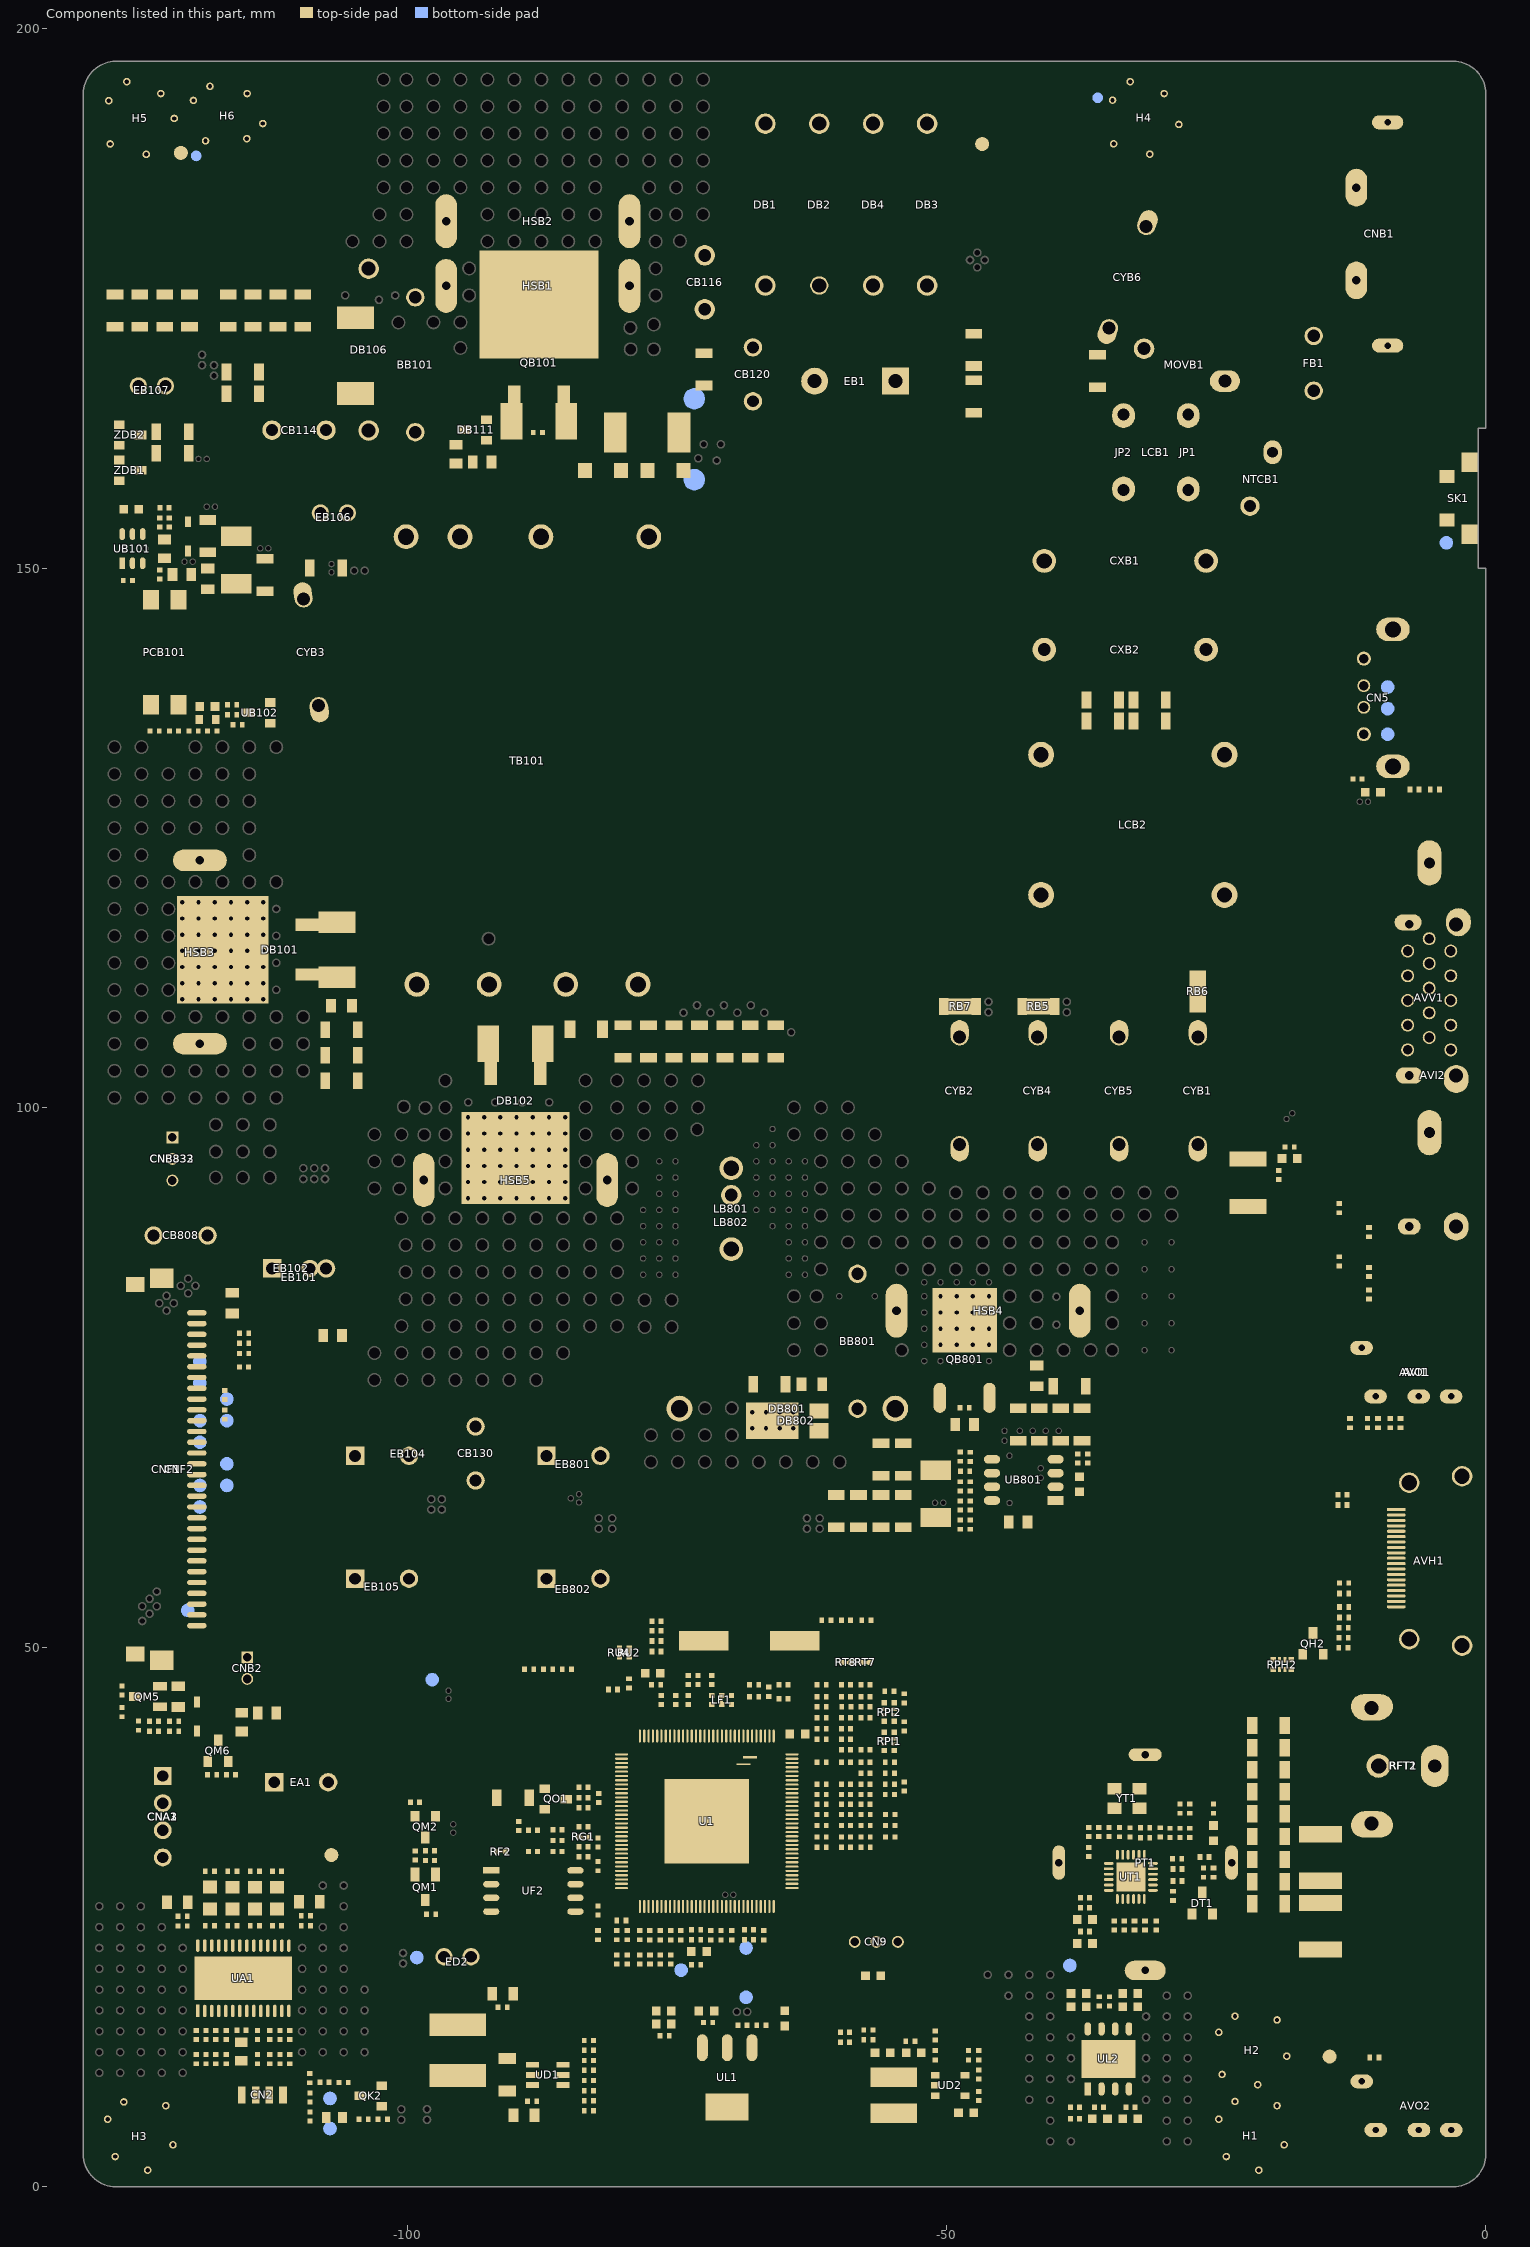
[diagram p0: the components of this part, seen from the top]
# Altium PCB MISC84438.PcbDoc (part 5 of 15)
Units mm, origin at the board's own origin, x right, y up, seen from the top; angles counter-clockwise.
Board outline 130 x 197 mm, 2 copper layers (TopLayer, BottomLayer), stack 1.571 mm thick; 574 components, 314 nets, 2636 pads, 811 vias.

## Footprints (in the part's own frame and the unit in brackets; to place one, negate y for a bottom-side part, rotate by r counter-clockwise, add the part's x,y. Pads: shape width x height; smd on the part's side, far side on the other; paste and mask are expansions set on the pad) (continued)
SIP3/2.0D-CP [mm] "捷仕泰/铭锋达;带扣插座与非带扣插座 兼容；15.07.11"
  rect 1.4x1.4 on Top Overlay: 0(-2,0)
  round 1.4 on Top Overlay: 0(0,0) 0(2,0)
  rect 1.1x1.1 hole 0.8: 1(-2,0)
  round 1.1 hole 0.8: 2(0,0) 3(2,0)
  silkscreen extent -4,-3.2 4,3.07, body extent -4,-3.2 4,1.8, height 6
SIP3H/2.0D-3 [mm] "捷仕泰：A2004AW-03-A1MA-P，带扣，加强筋"
  rect 1.6x1.6 on Top Overlay: 0(-2,0)
  round 1.6 on Top Overlay: 0(0,0) 0(2,0)
  rect 1.1x1.1 hole 0.8: 1(-2,0)
  round 1.1 hole 0.8: 2(0,0) 3(2,0)
  silkscreen extent -4.1,-7.95 4.1,1.5
SIP4/2.5D-2 [mm] "捷仕泰，A2502-04-A5WA-P（为保证与SIP4/2.54D-1兼容。改PIN间距为2.52mm，18.05.28）"
  rect 1.905x1.905 on Top Overlay: 0(-3.78,0)
  round 1.905 on Top Overlay: 0(-1.26,0) 0(1.26,0) 0(3.78,0)
  rect 1.651x1.651 hole 1.05: 1(-3.78,0)
  round 1.651 hole 1.05: 2(-1.26,0) 3(1.26,0) 4(3.78,0)
  silkscreen extent -6.4,-3.6 6.4,3
SIP4/2.54D-1 [mm] "捷仕泰/铭锋达"
  rect 1.905x1.905 on Top Overlay: 0(-3.78,0)
  round 1.905 on Top Overlay: 0(-1.26,0) 0(1.26,0) 0(3.78,0)
  rect 1.651x1.651 hole 1.05: 1(-3.78,0)
  round 1.651 hole 1.05: 2(-1.26,0) 3(1.26,0) 4(3.78,0)
  silkscreen extent -6.44,-3.5 6.44,2.5, body extent -6.35,-3.5 6.35,2.5, height 7
SIP4H/2.54D-2 [mm] "捷仕泰/铭锋达    SPEAKER"
  rect 1.905x1.905 on Top Overlay: 0(-3.78,0)
  round 1.905 on Top Overlay: 0(-1.26,0) 0(1.26,0) 0(3.78,0)
  rect 1.651x1.651 hole 1.05: 1(-3.78,0)
  round 1.651 hole 1.05: 2(-1.26,0) 3(1.26,0) 4(3.78,0)
  silkscreen extent -6.29,-7.2 6.29,0.89
SMD4532-1 [mm] "Brightking,4532-091-LF,气体放电管,雷电防护器件，17.06.12"
  rect 1.5x4 smd: 1(-2.15,0) 2(2.151,0)
  silkscreen extent -1.25,-1.79 1.23,1.71, body extent -2.41,-1.75 2.41,1.75, height 3
SO-8A [mm] "FLASH"
  rect 1.5x0.8 smd: 1(-2.95,1.905)
  oval 1.5x0.8 smd: 2(-2.95,0.635) 3(-2.95,-0.635) 4(-2.95,-1.905) 5(2.95,-1.905) 6(2.95,-0.635) 7(2.95,0.635) 8(2.95,1.905)
  silkscreen extent -4.71,-2.54 2,2.54, body extent -3.1,-2.5 3.1,2.5, height 1.76
SO-23 [mm] "双向二极管封装"
  rect 0.8x1 smd: 1(0.952,1.016) 3(-0.953,1.016)
  rect 0.8x1.1 smd: 2(0,-0.966)
  silkscreen extent -1.55,-0.86 1.55,0.36, body extent -1.5,-1.25 1.5,1.25, height 1.1
SOIC8 [mm] "W25X40BVSNIG/GD25Q32BSIG/GD25LQ16"
  rect 1.5x0.6 smd: 1(-3.9,1.905)
  oval 1.5x0.6 smd: 2(-3.9,0.635) 3(-3.9,-0.635) 4(-3.9,-1.905) 5(3.9,-1.905) 6(3.9,-0.635) 7(3.9,0.635) 8(3.9,1.905)
  silkscreen extent -5.71,-2.65 2.7,2.65, body extent -4.05,-2.69 4.05,2.69, height 2.17
SOP8/1.27-3 [mm] "LEADCHIP;LC1118;14-05-09"
  rect 1.238x0.6 smd: 1(-2.783,1.905)
  oval 1.238x0.6 smd: 2(-2.783,0.635) 3(-2.783,-0.635) 4(-2.783,-1.905) 5(2.783,-1.905) 6(2.783,-0.635) 7(2.783,0.635) 8(2.783,1.905)
  rect 3.5x5 smd paste-3 mask-3: EPAD(0,0)
  silkscreen extent -3.31,-2.5 4.16,3.42, body extent -3.1,-2.5 3.1,2.5, height 1.76
SOT-23 [mm]
  rect 0.8x1 smd: B(0.952,1.016) E(-0.953,1.016)
  rect 0.8x1.1 smd: C(-0.013,-0.966)
  silkscreen extent -1.55,-0.81 1.55,0.36, body extent -1.5,-1.25 1.5,1.25, height 1.1
SOT-23-1 [mm]
  rect 0.8x1.1 smd: D(0,-1.15)
  rect 0.8x1.27 smd: G(0.95,1.2) S(-0.95,1.2)
  TopLayer pour cut-out: -1.583,0.903 -1.583,-0.905 1.587,-0.905 1.587,0.903
  silkscreen extent -1.55,-1.05 1.55,0.33, body extent -1.52,-1.48 1.52,1.48, height 1.25
SOT-23-5 [mm] "LPW5206(1.295mm)"
  rect 0.6x0.8 smd: 1(-0.95,-1.375) 2(0,-1.375) 3(0.95,-1.375) 4(0.95,1.375) 5(-0.95,1.375)
  silkscreen extent -1.5,-2.49 1.5,0.85, body extent -1.5,-0.85 1.5,0.85, height 1.45
SOT-23-6 [mm] "RICHTEK RT9266//RT7295A(1mm)"
  rect 0.55x1.2 smd: 1(-0.95,-1.4) 2(0,-1.4) 3(0.95,-1.4) 4(0.95,1.4) 5(0,1.4) 6(-0.95,1.4)
  silkscreen extent -2.4,-1.88 1.55,0.9, body extent -1.55,-0.9 1.55,0.9, height 1.3
SOT-23-RAK [mm] "TL431G-AE2-R(UTC)"
  rect 0.8x1.1 smd: A(0.013,0.966)
  rect 0.8x1 smd: K(0.953,-1.016) R(-0.953,-1.016)
  silkscreen extent -1.52,-0.36 1.52,0.86, body extent -1.5,-1.25 1.5,1.25, height 1.1
SOT-26 [mm] "LD7536R"
  rect 0.5x1.1 smd: 1(0.95,1.35)
  oval 0.5x1.1 smd: 2(0,1.35) 3(-0.95,1.35) 4(-0.95,-1.35) 5(0,-1.35) 6(0.95,-1.35)
  silkscreen extent -1.55,-2.54 2.29,1.76, body extent -1.55,-0.9 1.55,0.9, height 1.45
SOT-223 [mm]
  oval 1x2.5 smd: 1(-2.3,-2.75) 2(0,-2.75) 3(2.3,-2.75)
  rect 4x2.5 smd: 4(0,2.75)
  TopLayer pour cut-out: 2.3,-1.188 2.3,-4.312 -2.345,-4.312 -2.64,-4.253 -2.891,-4.086 -3.058,-3.835 -3.117,-3.54 -3.117,-3.54 -2.299,-3.54 -2.299,-1.956 -3.124,-1.956 -3.066,-1.662 -2.899,-1.413 -2.65,-1.247 -2.356,-1.188 -2.356,-1.188
  silkscreen extent -3.45,-2.75 3.45,2.81, body extent -3.35,-3.3 3.35,3.4, height 1.7
SSOP28/0.65-5 [mm] "TI;TPA3140D2PWPR;15.07.08"
  rect 1.15x0.34 smd: 1(-3.025,4.225)
  oval 1.15x0.34 smd: 2(-3.025,3.575) 3(-3.025,2.925) 4(-3.025,2.275) 5(-3.025,1.625) 6(-3.025,0.975) 7(-3.025,0.325) 8(-3.025,-0.325) 9(-3.025,-0.975) 10(-3.025,-1.625) 11(-3.025,-2.275) 12(-3.025,-2.925) 13(-3.025,-3.575) 14(-3.025,-4.225) 15(3.025,-4.225) 16(3.025,-3.575) 17(3.025,-2.925) 18(3.025,-2.275) 19(3.025,-1.625) 20(3.025,-0.975) 21(3.025,-0.325) 22(3.025,0.325) 23(3.025,0.975) 24(3.025,1.625) 25(3.025,2.275) 26(3.025,2.925) 27(3.025,3.575) 28(3.025,4.225)
  oct 1.05x1.318 on Top Paste mask+0.076: EPAD(-0.675,2.427) EPAD(-0.675,0.809) EPAD(-0.675,-0.809) EPAD(-0.675,-2.427) EPAD(0.675,2.427) EPAD(0.675,0.809) EPAD(0.675,-0.809) EPAD(0.675,-2.427)
  oct 1.05x1.318 on Top Solder mask+0.076: EPAD(-0.675,2.427) EPAD(-0.675,0.809) EPAD(-0.675,-0.809) EPAD(-0.675,-2.427) EPAD(0.675,2.427) EPAD(0.675,0.809) EPAD(0.675,-0.809) EPAD(0.675,-2.427)
  rect 4x9 smd paste-5 mask-5: EPAD(0,0)
  silkscreen extent -4.65,-4.9 4.64,5.31, body extent -2.25,-4.9 2.25,4.9, height 1.2
T-13.2×12.4×7.7-F14.5 [mm] "LHD;13.2×12.4×7.7-F14.5 中心出口高度6.3mm；160713(18.08.30 优化短槽孔）"
  oval 2.5x4.1 on Top Overlay paste-4 mask-4: 0(-5.5,6.1) 0(5.5,6.1)
  round 2.3 on Top Overlay: 0(0,5.45)
  oval 4.1x2.7 on Top Overlay paste-4 mask-4: 0(0,0.25)
  round 2.1 hole 1.4: 1(0,5.45)
  oval 2.3x3.9 hole 1 slot 2.6 at 90 deg: 2(-5.5,6.1) 4(5.5,6.1)
  oval 3.9x2.5 hole 1.2 slot 2.6 at 0 deg: 3(0,0.25)
  KeepOutLayer pour cut-out: -1.438,5.45 -1.329,4.902 -1.019,4.438 -0.555,4.128 -0.007,4.019 -0.007,4.019 0.541,4.128 1.005,4.438 1.315,4.902 1.424,5.45 1.424,5.45 1.315,5.998 1.005,6.462 0.541,6.772 -0.007,6.881 -0.007,6.881 -0.555,6.772 -1.019,6.462 -1.329,5.998 -1.438,5.45
  silkscreen extent -6.3,0 6.3,7.9, body extent -7.55,-35.2 7.55,7.7, height 13.85
T/EQ2914*9-1 [mm] "SYEQ2914Z-T012021A-YX,17.10.10"
  round 2.5 on Top Overlay: 0(-16.1,-6.25) 0(-16.1,1.25) 0(-16.1,-11.25) 0(-16.1,11.25) 0(25.4,10.25) 0(25.4,-10.25) 0(25.4,-3.55) 0(25.4,3.55)
  round 2.3 hole 1.5 mask+0.076: 1(-16.1,11.25) 3(-16.1,1.25) 4(-16.1,-6.25) 5(-16.1,-11.25) 6(25.4,-10.25) 7(25.4,-3.55) 8(25.4,3.55) 9(25.4,10.25)
  silkscreen extent -18.7,-15.5 26.6,15.5
TO-252-GDS [mm] "SC08440  IRLR024N"
  rect 6x6 smd: D(0,0)
  oval 1.143x2.794 smd: G(-2.3,-7.2) S(2.3,-7.2)
  silkscreen extent -3.4,-5.64 3.4,3.4, body extent -3.4,-7.75 3.4,2.45, height 2.5
TP [mm] "TEST POINT"
  round 1.27 smd paste-1.27: 1(0,0)
TP-10 [mm] "TEST POINT;1mm"
  round 1 smd: 1(0,0)
TP-TDT [mm] "电源放电测试点，间隔7.5mm"
  round 2 smd paste-2: 1(-3.75,0) 2(3.75,0)
  silkscreen extent -5.75,-2 5.75,2
TP_BL [mm] "TEST POINT,专用背光测试点"
  round 1.27 smd paste-1.27: 1(0,0)
  silkscreen extent -6.4,-0.97 0.95,0.96
USB-HD-30 [mm] "广业，USB-20161027-0011，17.07.27"
  oval 2.4x3.3 on Top Overlay: 0(-6.35,8.11) 0(6.35,8.11)
  round 1.5 on Top Overlay: 0(-3.37,10.81) 3(3.63,10.81)
  round 1.3 hole 0.9: 1(-3.37,10.81) 4(3.63,10.81)
  round 1.4 on Top Overlay: 1(-0.87,10.81) 2(1.13,10.81)
  round 1.2 hole 0.9: 2(-0.87,10.81) 3(1.13,10.81)
  oval 2.2x3.1 / inner oval 2.2x3.1 / far side oval 2.9x3.8 hole 1.5 slot 2.4 at 90 deg: 5(6.35,8.11) 6(-6.35,8.11)
  KeepOutLayer pour cut-out: -3.063,12.516 -3.825,12.38 -4.475,11.958 -4.911,11.318 -5.064,10.559 -5.064,10.559 -4.765,9.743 -4.118,9.161 -3.275,8.95 -3.275,8.95 1.967,8.95 2.407,9.037 2.781,9.287 3.03,9.66 3.118,10.101 3.118,10.101 3.118,11.085 3.009,11.632 2.699,12.097 2.234,12.407 1.686,12.516 1.686,12.516
  silkscreen extent -6.65,-0.06 6.65,12, body extent -7.4,-2 7.4,11.9, height 9.4
VR(13*5)-V-7.5 [mm] "为勤,VARISTOR,17.01.04修改为椭圆孔;160105更新椭圆孔"
  oval 2.8x2 hole 1.2 slot 2 at 0 deg: 1(3.75,-1.5)
  round 1.9 hole 1.2: 2(-3.75,1.5)
  round 2.1 on Top Overlay: 2(-3.75,1.5)
  oval 3x2.2 on Top Overlay: 2(3.75,-1.5)
  silkscreen extent -6.65,-2.5 6.42,2.5, body extent -6.5,-2.75 6.5,2.75, height 15.5
XTAL-S-1 [mm] "假贴晶振（威特电子）"
  rect 4.6x1.8 smd: 1(-4.207,0) 2(4.207,0)
  silkscreen extent -5.8,-2.41 5.8,2.41, body extent -6.4,-2.36 6.39,2.38, height 5
XTAL-S-10 [mm] "铜陵晶威特；SMD3225"
  rect 1.3x1.1 smd: 1(-1.15,-0.9) 2(1.15,-0.9) 3(1.15,0.9) 4(-1.15,0.9)
  silkscreen extent -2.88,-1.3 1.65,1.3, body extent -1.65,-1.3 1.65,1.31, height 0.8

## Part data
AVH1: library part XXX.XXX.0001809-D, "HDMI terminal,HDMI Jack,H,Block up,SMD,51U019S-313HFN-E-R-F,FREEPORT-D"
AVI1 AVO1 AVO2: library part "耳机端子,Earphone Jack,H,Φ3.6,CH5.5,Black,DIP-DLMI"
AVI2: library part XXX.XXX.0003577-DLMI, "RCA terminal,RCA Jack,AV3,H,Red, White, Yellow,CH5.5,D14,Seal,DIP,RC075-F03L3BY-L,YUQIU-DLMI"
AVV1: library part WLHD-051A-DLMI-DB15, "CN-DB15-horizontal-#-#-#"
BB101: library part φ3.5×6.0×0.65mm-CP(编带/秀益达)-DAI, "Through-hole ferrite bead"
BB801: library part φ3.5×6.0×0.65mm-CP(编带/秀益达)-DLAI, "Through-hole ferrite bead"
CA4 CA5 CA10 CA16 CA17 CA25 CA27 CA29 CB103 CF29 CF30 CI10 CI11: library part 1000pF-0402-X7R-±10%-50V-D
CA6 CA8 CA20 CA21: library part 0.22uF-0402-X5R-±10%-16V-D
CA7 CA12 CA13 CA22: library part 0.22uF-0402-Y5V-+80%-20%-16V-D
CA15 CA18 CD17 CH15: library part 1uF-0402-X5R-±20%-16V-D
CA23 CA24 CA28 CD12 CD16 CF2 CF7 CF8 CF9 CF10 CF12 CF13 CF14 CF17 CG1 CH8 CH9 CI3 CI4 CI6 CI7 CK4 CK10 CL2 CL3 CM1 CM2 CM4 CT1 CT5 CT9 CT11 CT18 CT20 CT21 CT23 CT25 CT27 CU2 CU3: library part 0.1uF-0402-Y5V-+80%-20%-16V-D
CA31 CA32 CD11 CD14 CD15 CF5 CF15 CF22 CF28 CF37 CL1 CL4 CL5 CL7 CL8 CL11 CL12 CL14 CL15 CT3 CT6 CU1 CU4: library part 10uF-0603-X5R-±20%-6.3V-D
CB101 CB803 CB813 CO3 CO5 CO9: library part 100pF-0402-NPO-±5%-50V-D
CB102 CB109: library part 0.1uF-0603-X7R-±10%-50V-D, "CAP"
CB110 CB125 CB806: library part 1000pF-0402-X7R-±10%-50V-D, "CAP"
CB113 CB131: library part 220PF-0805-NPO-±10%-200V-D, "CAP"
CB114: library part C242G472J20A201(编带/法拉)-DAI, "CAP"
CB116: library part 004.003.0001889-DHAI, "Ceramic capacitor,CAP CD,1KV,100pF,±5%,SL,OK,5.0mm,DIP,TP,TDK-DHAI"
CB117: library part 1000pF-0805-NPO-±10%-200V-D, "CAP"
CB118: library part "陶瓷电容,CAP MC,1KV,4700pF,±10%,X7R,1206,SMD,TP,ISND-D"
CB120 CB130 CB808: library part 004.003.0001665, "Ceramic capacitor,CAP CD,1KV,4700pF,±20%,Y5U,K,5.0mm,DIP,TP,Walsin-DHAI"
CB801: library part 1uf-0603-X7R-±10%-25V-D
CB804: library part 4700pF-0402-X7R-±10%-50V-D
CB805 CD2: library part 0.1uF-0402-X7R-±10%-16V-D
CB809 CB810: library part 004.003.0001392, "Ceramic capacitor,CAP MC,500V,47pF,±5%,NPO,0805,SMD,TP,WALSIN-D"
CB812: library part 0.033uF-0402-X7R-±10%-16V-D
CD1 CD22 CM5: library part 10uF-0805-X5R-±20%-16V-D
CD13: library part 3300pF-0402-X7R-±10%-50V-D
CD19 CD21 CL6 CL9 CL10 CL13 CM3: library part 0.1uF-0402-X5R-±20%-16V-D
CD20: library part 22pF-0402-NPO-±5%-50V-D
CD41: library part 10uF-1206-X5R-±10%-16V-D
CF1 CF4 CH10 CT7 CT8: library part 33pF-0402-NPO-±5%-50V-D
CF6 CF16 CF18 CF19 CF20 CF21 CF23 CF24 CF25 CO1 CO4: library part 1uF-0402-X5R-±20%-6.3V-D
CF26 CF31 CF34 CI1 CI8 CV1 CV3 CV7: library part 0.047uF-0402-X7R-±10%-16V-D
CF33 CF35: library part 5pF-0402-NPO-±5%-50V-D
CF38: library part 0.1uF-0402-X5R-±20%-16V-
CF39 CF40 CV9 CV10: library part 30pF-0402-NPO-±5%-50V-D
CK2: library part 0.01uF-0402-X7R-±10%-50V-D
CK6: library part 10pF-0402-NPO-±5%-50V-D
CM7 CT12 CT19: library part 0.022uF-0402-X7R-±10%-16V-D
CN2: library part 红外接收三极管,Phototransistor,NPN,6.8×3×3.2mm,SMD,HS75438D,VISHAY-D
CN5: library part PKG-003212/P000071027, "USB terminal,USB2.0,H,Single,Block up,DIP,U250FD004S1549BY-DLMI"
CN9: library part 3PIN-2.0-D-H-G-带扣-DHMI
CNA1: library part 4PIN-2.54-D-H-G-DHMI
CNA2: library part XXX.XXX.0000738-DLMI-SPEAKER, "Connector socket,connect jack,4Pin,D2.50,L,L=2.8mm,DIP,CNJST-DLMI"
CNA3: library part 4PIN-2.54-D-H-G-带扣-B-DHMI
CNB1: library part "连接插座,connect jack,2Pin,D8.6,L,SNAP,Fool-proofing,Black,L=4.0mm,DIP,YQ-DLMI", "AC socket, side exit (figure-eight)"
CNB2: library part XXX.XXX.0001753, "Connector socket,connect jack,2Pin,D2.0,D,L=2.8mm,DIP,AMA-DHMI"
CNB832: library part XXX.XXX.0001754, "Connector socket,connect jack,3Pin,D2.0,D,L=2.8mm,DIP,AMA-DHMI"
CNB833: library part 3PIN-2.0-L-H-G-带扣-带台阶-J-DLMI
CNF1: library part XXX.XXX.0004205-D, "FFC socket,FFC connector,30Pin,D1.0,Bottom,lock,SMD,F10033FA030M1WL,CT-D"
CNF2: library part 196161-30041-3, "CN-FFC socket-flip cover"
"Conformal Coating": library part 三防漆,25kg/Can,Peters
CT10 CT24: library part 56pF-0402-NPO-±5%-50V-D
CT13: library part 1.8pF-0402-NPO-±0.25pF-50V-D
CT14 CT15: library part 8pF-0402-NPO-±5%-50V-D
CT17: library part 120pF-0402-NPO-±5%-50V-D
CT26: library part 330pF-0402-NPO-±5%-50V-D
CT29: library part 6800pF-0402-X7R-±10%-50V-D
CT40: library part 4700pF-1206-X7R-±10%-1000V-D
CT41 CT42 CT43 CT44 CT45 CT46 CT47 CT48: library part 1000pF-1206-X7R-±20%-2000V-D
CXB1: library part "X电容,CAP X2,MP,275VAC,0.47uF,±10%,S,15mm-Mini,PC,DIP,BM-DHMI", "CAP"
CXB2: library part PX104K3ID19H200D9R(凯励)-DHMI, "X capacitor"
CYB1 CYB2 CYB3 CYB4 CYB5 CYB6: library part "Y电容,CAP Y1,CD,470pF,400VAC,±20%,KS,10mm,Y5U,DIP,Walsin-DHMI", "Y1 capacitor"
DB1 DB2 DB3 DB4 DB106: library part RL207G(编带/GOOD-ARK)-DLAI, "Diode"
DB101: library part 004.005.0000140-D, "Rectifier diode,DIO SI D1,10A,150V,TO-263,SMD,MBRB10150CT,GOOD-ARK-D"
DB102: library part 004.005.0000473, "Rectifier diode,DIO FRD D1,10A,400V,TO-263,SMD,MURB1040S,GOOD-ARK-D"
DB103: library part "整流二极管,DIO SI S,3A,1000V,SMC,SMD,HS3M R6,TSC-D", "Diode"
DB104 DB804: library part M7(WEJ)-D, "Diode"
DB109 DB110: library part "整流二极管,DIO FRD S,1.2A,800V,eSGA,SMD,R12K,GOOD-ARK-D"
DB111 ZDB2: library part LBAV70LT1G(LRC)-D, "Diode"
DB112: library part BAV21WS-D, "Diode"
DB801: library part "肖特基二极管,DIO SBD S,3A,150V,DO-201AD,DIP,SR315 A0G,TSC-DLMI", "Diode"
DB802: library part TSPB5H150S-D, "Diode"
DH2 DH3 DH6 DH7 DH8 DH9 DI1 DI2 DI3 DI5 DK1 DO1 DO2 DO3 DT2 DT3 DU1 DU2 DU3 DU4 DV1 DV2: library part AVLC18S02003-D
DK20: library part WEJT61RC-871-红色-D
DM1: library part 1N4148WS-D
DT1: library part BAV99-BR-D
EA1: library part 470uF-25V-±20%-10×12-105℃-YE-编带-F=5.0(Elite)-DHAI, "Electrolytic"
EB1: library part 100uF-450V-±20%-18×41-105℃-KS-折脚开槽(CapXon)-S对策-DLMI, "Electrolytic"
EB101: library part 470uF-25V-±20%-10×12.5-105℃-GF-编带-F=5.0(CapXon)-DHAI, "Electrolytic"
EB102: library part 270uF-16V-±20%-8×11-105℃-RP-短脚-F=3.5(Elite)-DHMI, "CAP"
EB104 EB105: library part 100uF-63V-±20%-10×12.5-105℃-GF-编带-F=5.0(CapXon)-DHAI, "Electrolytic"
EB106 EB107: library part 10uF-50V-±20%-5×11-105℃-GH-编带-F=2.5(CapXon)-DHAI, "Electrolytic"
EB801 EB802: library part 47uF-100V-±20%-10×12-105℃-EV-编带-F=5.0(Elite)-DHAI, "Electrolytic"
ED2: library part 470uF-10V-±20%-6.3×11-105℃-黑底白字-编带-F=2.5-XF-DHAI, "Electrolytic"
F1: library part MSMD110-D, "FUSE"
F2: library part 5R1ohm-0402-±5%-1/16W-D
FB1: library part 004.026.0000010-DHMI, "Slow-blow fuse,FUSE T,P,3.15A,250VAC,8.5×4.0×8mm,DIP,TP,Walter-DHMI"
GDT1 GDT2: library part 004.005.0000675, "Gas discharge tube,GDT,700V,2000A,TP,4.5*3.2mm,SMD,4532-091-LF,Brightking-D"
GL1: library part 005.002.0000011, "Silicone,0.2g,general,60,white,SLD-8854W,XY-DHMI"
H1 H2 H3 H4 H5 H6: library part "Location hole-D"
HS1: library part 14×14×06-THD-HS, "SMD heatsink"
HSB1 HSB2 HSB3 HSB4 HSB5: library part 17.5×14.5×0.5-本色-Cu-MRD-D, "Heatsink"
JP1 JP2: library part 004.002.0002101-DLAI, "Jumper,RES JUMP,0.6,7.0mm,DIP-DLAI"
LB801: library part SYDR1212-L003-EDL-DHMI, "I-type inductor"
LB802: library part 差模电感,Inductor,DR12×14,68uH,0.45,20Ts,H13.5MAX,SYDR1214-L068uA,DIP,Soldier-DHMI, "I-type inductor"
LBA1 LBA2 LBA3 LBA4: library part 300ohm-2500mA-0805-D
LCB1: library part 004.004.0002338-DHMI, "Common-mode choke,Common Choke,T9×5×3,230uH MIN,0.45×1P,7.5Ts,H14.0MAX,SYT09-L230uA,DIP,CK-DHMI"
LCB2: library part 004.004.0002597-DHMI, "Common-mode choke,Common Choke,UC1614,10.5mH±10%,0.15×1.0mm,48Ts,H14.0MAX,SYUC16-L10.5mA,DIP,CH-DHMI"
LD2: library part SLN43T-6R8M-D
LD3: library part SWPA6045S4R7MT-D
LF1 RF2 RG1 RT7 RT8 RU2 RU4: library part 0ohm-0402-PCB-D, "0ohm-0402-PCB-D"
LF6 RA14 RD2 RD15 RH1 RH2 RI13 RI14 RI15 RL1 RL2 RO13 RO14 RO15 RR1: library part 0ohm-0402-±5%-1/16W-D
LT1: library part SDCL1005C68NJTDF(68nH-0402±5%-C)-D
LT2 LT6 LT8: library part 1Kohm-0402-±25%-D
LT3: library part 2.2nH-0402-±0.3nH-1/4-D
LT9: library part SDCL1005CR33JTDF-D
LT10: library part SDCL1608CR22JT(F)-D
LT11: library part SDCL1005CR27JTDF(顺络)-D
LT12: library part GZ1005U121CTF(120ohm-500mA)-D
M1 M2 M3 M4: library part MARK-D
MOVB1: library part TVR10561KSW(为勤)-DHMI, "Varistor"
NTCB1: library part SCK102R55AMBY502(短脚/为勤)-DHMI, "Thermistor"
PCB101: library part LTV-817S-TA-B(光宝)-DMI, "Optocoupler"
PT1: library part 20.3×16.3×6-LHD(带封口)-DMI
PWM_REF TB-GND1 TB-GND2: library part TEST
QB101: library part 004.007.0000227-D, "MOSFET,NMOS,13.7A,650V,0.22ohm@ID=6.9A@VGS=10V,D2PAK,TK14G65W,TOSHIBA-D"
QB801: library part AOD4454(AOS)-D, "N Channel Single MOSFET"
QH2 QK2: library part MMBT3904(f≥350MHz)-D-NPN, "Q-NPN-#-#-#"
QM1: library part WPM2341A-3/TR-D
QM2 QM6 QO1: library part LMBT3904LT1G-D-NPN, "Q-NPN-#-#-#"
QM5: library part WPM3407C-3/TR-D
R1 R2 R3 RF3 RF8 RF9 RF22 RF26 RK15 RK18 RT3 RT4: library part 4K7ohm-0402-±5%-1/16W-D
R5V R12V: library part 0ohm-0805-±5%-1/8W-D
RA1 RA8 RF10 RF11 RK13 RO9 RV10 RV12: library part 100ohm-0402-±5%-1/16W-D
RA2 RA15: library part GND
RA3: library part 10ohm-0805-±5%-1/8W-D
RA4 RM7 RO3 RO7: library part 47Kohm-0402-±5%-1/16W-D
RA5 RA21: library part 180ohm-0402-±5%-1/16W-D
RA11: library part 12Kohm-0402-±5%-1/16W-D
RA12: library part 9K1ohm-0402-±5%-1/16W-D
RB1 RB2 RB3 RB4: library part 1M2ohm-1206-±5%-1/4W-D, "RES"
RB5 RB6 RB7: library part 0ohm-1206-PCB-D, "0ohm-1206-PCB-D"
RB8 RB110 RB111 RB116 RB117 RB118 RB119 RB130 RB810 RB812: library part 10ohm-1206-±5%-1/4W-D, "RES"
RB101 RB102: library part 330Kohm-1206-±5%-1/4W-D, "RES"
RB103 RD16: library part 6K8ohm-0402-±1%-1/16W-D
RB104: library part 27Kohm-0402-±1%-1/16W-D
RB105: library part 510ohm-0402-±1%-1/16W-D
RB106: library part 68ohm-0805-±5%-1/8W-D
RB107 RB807: library part 20ohm-0805-±5%-1/8W-D, "RES"
RB109 RB133 RB808: library part 10Kohm-0402-±1%-1/16W-D
RB112 RB113 RB140: library part 51Kohm-0805-±1%-1/8W-D, "RES"
RB114: library part 4R7ohm-1206-±1%-1/4W-D, "RES"
RB124 RB125 RB126 RB127 RB162 RB163 RB164 RB165: library part 68ohm-1206-±5%-1/4W-D, "RES"
RB128 RB129: library part 47ohm-1206-±5%-1/4W-D, "RES"
RB131: library part 2Kohm-0603-±5%-1/10W-D
RB132 RB806: library part 1Kohm-0402-±1%-1/16W-D
RB134: library part 4K7ohm-0402-±1%-1/16W-D, "RES"
RB135: library part 18Kohm-0402-±1%-1/16W-D, "RES"
RB148: library part 004.002.0001050, "Thick-film resistor,RES,2W,0.22ohm,±5%,2512,SMD-D"
RB150 RB151 RB152 RB153 RB154 RB155 RB156 RB157: library part 100Kohm-1206-±5%-1/4W-D, "RES"
RB158: library part 3Kohm-0402-±1%-1/16W-D
RB803: library part 9K1ohm-0402-±1%-1/16W-D
RB804 RH10 RH11 RK20 RM3 RM4 RO6 RT2 RT18 RV13 RV14: library part 10Kohm-0402-±5%-1/16W-D
RB805: library part 100ohm-0402-±5%-1/16W-D, "RES"
RB813: library part 100ohm-0402-±1%-1/16W-D
RB814 RB835: library part 004.002.0001261, "Thick-film resistor,RES,1/4W,510Kohm,±1%,1206-Auto,SMD-D"
RB816: library part 33ohm-0805-±5%-1/8W-D
RB818 RB819 RB820 RB821: library part 0R3ohm-1206-±5%-1/4W-D
RB837 RB838: library part 1R5ohm-1206-±1%-1/4W-D, "RES"
RB839: library part 2R2ohm-1206-±1%-1/4W-D, "RES"
RB840: library part 1R6ohm-1206-±1%-1/4W-D, "RES"
RD6: library part 12Kohm-0402-±1%-1/16W-D
RD7: library part 12K4ohm-0402-±1%-1/16W-D
RD8: library part 68Kohm-0402-±1%-1/16W-D
RD13: library part 39Kohm-0402-±1%-1/16W-D, "RES"
RD14 RM2: library part 100Kohm-0402-±5%-1/16W-D
RD88 RF1: library part 1Mohm-0402-±5%-1/16W-D
RF12 RF16 RF19: library part 68ohm-0402-±5%-1/16W-D
RF14 RF15 RO4 RO8: library part 200Kohm-0402-±5%-1/16W-D
RF20: library part 100ohm-0402-±5%-1/16W-
RF21 RF23 RF25 RF27: library part 1Kohm-0402-±5%-1/16W-
RF24 RH14 RK3 RK16 RK21 RO10: library part 1Kohm-0402-±5%-1/16W-D
RFT1: library part "RF头,RF JACK,H,F,T14.5,CH6.3,without pipe,12.4×13.2×7.7mm,DIP,LHD-DLMI", "T-F-6.3mm-#-#"
RFT2: library part "RF头,RF JACK,H,IEC,T14.5,CH6.3,12.4×13.2×7.7mm,DIP,LHD-020组件,LHD-DLMI", "T-IEC-6.3mm-#-#"
RH13 RH28 RH29 RT9: library part 220ohm-0402-±5%-1/16W-D
RI2 RI8 RL4: library part 150ohm-0402-±1%-1/16W-D
RI3 RI9 RO12 RV2 RV5 RV11: library part 75ohm-0402-±5%-1/16W-D
RK1: library part 22ohm-0402-±5%-1/16W-D
RK4 RK6: library part 4K7ohm-0402-±1%-1/16W-D
RL5: library part 91ohm-0402-±1%-1/16W-D
RM1 RM5 RM6 RM8: library part 4k7ohm-0402-±5%-1/16W-D
RM10: library part 2K2ohm-0402-±5%-1/16W-D
RO1 RO5: library part 510ohm-0402-±5%-1/16W-D
RO2: library part 100ohm-1206-±5%-1/4W-D, "RES"
RPH2 RPI1 RPI2: library part 4*100ohm-0402-±5%-1/16W-D
RT5 RT6 RV1 RV3 RV9: library part 33ohm-0402-±5%-1/16W-D
RT11: library part 1K8ohm-0402-±5%-1/16W-D
SK1: library part TS06PW0-G35F(YF)-D
TB101: library part 004.004.0002082, "Transformer,EQ2914,270uH,0.35×2P,25Ts,H14.5MAX,SYEQ2914Z-T012021A (BLACK),DIP,YX-DHMI"
TP-TDT: library part TEST, "TEST"
U1: library part TSU69ZR-D
UA1: library part "音频功放,IC Audio AMP,Class D,2×9W@13V@8ohm,HTSSOP28,SMD,TPA3136D2,TI-D"
UB101: library part LD7537RGL(通嘉)-D, "IC"
UB102: library part AZ431AN-ATRE1(BCD)-D, "SMD 431 (shunt regulator)"
UB801: library part OB3350CPA(OB)-D, "IC"
UD1: library part "DC-DCоƬ,IC DCDC,Syn,3A,17V,650kHz,SOT-23,SMD,SN1501019DDCR,TI-D"
UD2: library part "DC-DCоƬ,IC DCDC,Syn,1.2A,7.0V,1.5MHz,SOT23-5,SMD,LC2127CB5TR,Leadchip-D"
UF2: library part "SPI FLASH оƬ,IC SPI FLASH,32Mb,SOIC8,SMD,GD25Q32CSIG,GigaDevice-D"
UL1: library part LC1117CLTR18-D
UL2: library part LC1118-D
UT1: library part R840-D
YF1: library part 24MHz-±20PPM-20PF-HC-49S-SMD-D
YT1: library part 004.009.0000056, "Passive standard-package crystal oscillator,SPXO,24MHz,±20ppm,16pF,3.2×2.5,SMD,SMD3225 24.000MHZ,JWT-D"
ZDB1: library part LBZX84C24LT1G(LRC)-D, "Diode"
用于U1上方: library part Φ12mm×12mm-黑色-125度(UL认证)-D